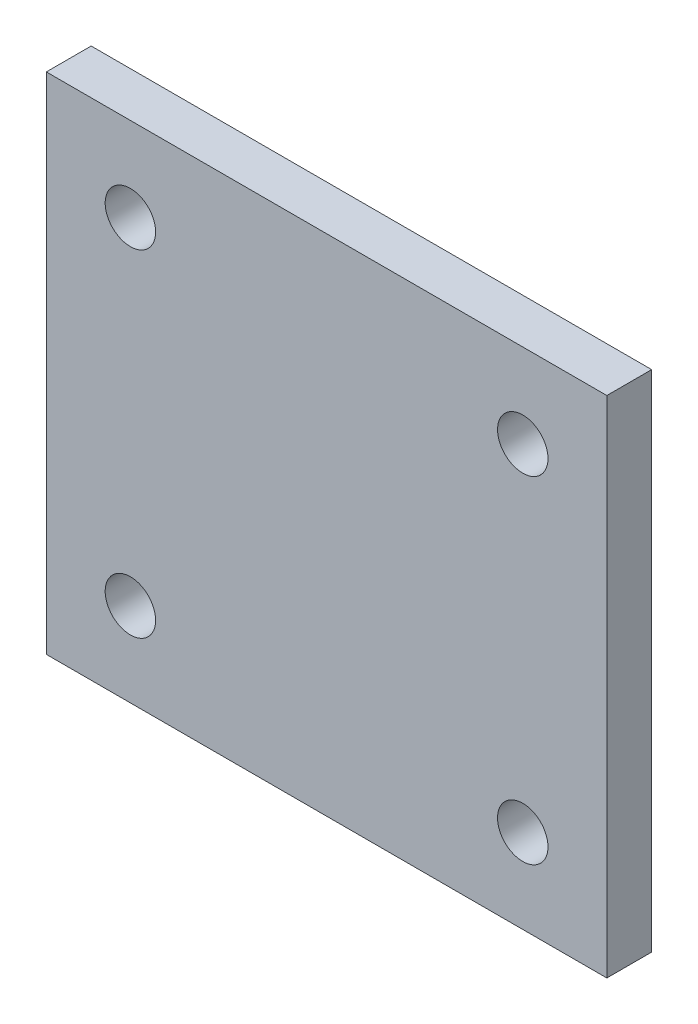
SolidWorks part; units mm, degrees
ref_plane "前视基准面" through (0, 0, 0) normal (0, 0, 1) x (1, 0, 0)
ref_plane "上视基准面" through (0, 0, 0) normal (0, 1, 0) x (1, 0, 0)
ref_plane "右视基准面" through (0, 0, 0) normal (1, 0, 0) x (0, 0, -1)
other "Configuration Table"
sketch "草图1" plane through (0, 0, 0) normal (0, 0, 1) x (1, 0, 0)
  line L0 (-50, -45) -> (50, -45)
  line L1 (50, -45) -> (50, 45)
  line L2 (50, 45) -> (-50, 45)
  line L3 (-50, 45) -> (-50, -45)
  point P0 (0, 0)
  dimension "D1" = 50
  dimension "D2" = 100
  dimension "D3" = 45
  dimension "D4" = 90
extrude "凸台-拉伸1" add sketch "草图1" against normal mid plane 8
sketch "草图2" plane through (0, 0, 0) normal (0, 0, 1) x (1, 0, 0)
  circle A0 centre (-35, -30) radius 4.5
  circle A1 centre (35, -30) radius 4.5
  circle A2 centre (-35, 30) radius 4.5
  circle A3 centre (35, 30) radius 4.5
  point P0 (0, 0)
  dimension "D1" = 9
  dimension "D2" = 9
  dimension "D3" = 9
  dimension "D4" = 9
  dimension "D5" = 35
  dimension "D6" = 70
  dimension "D7" = 30
  dimension "D8" = 60
extrude "切除-拉伸1" cut sketch "草图2" against normal mid plane 28
